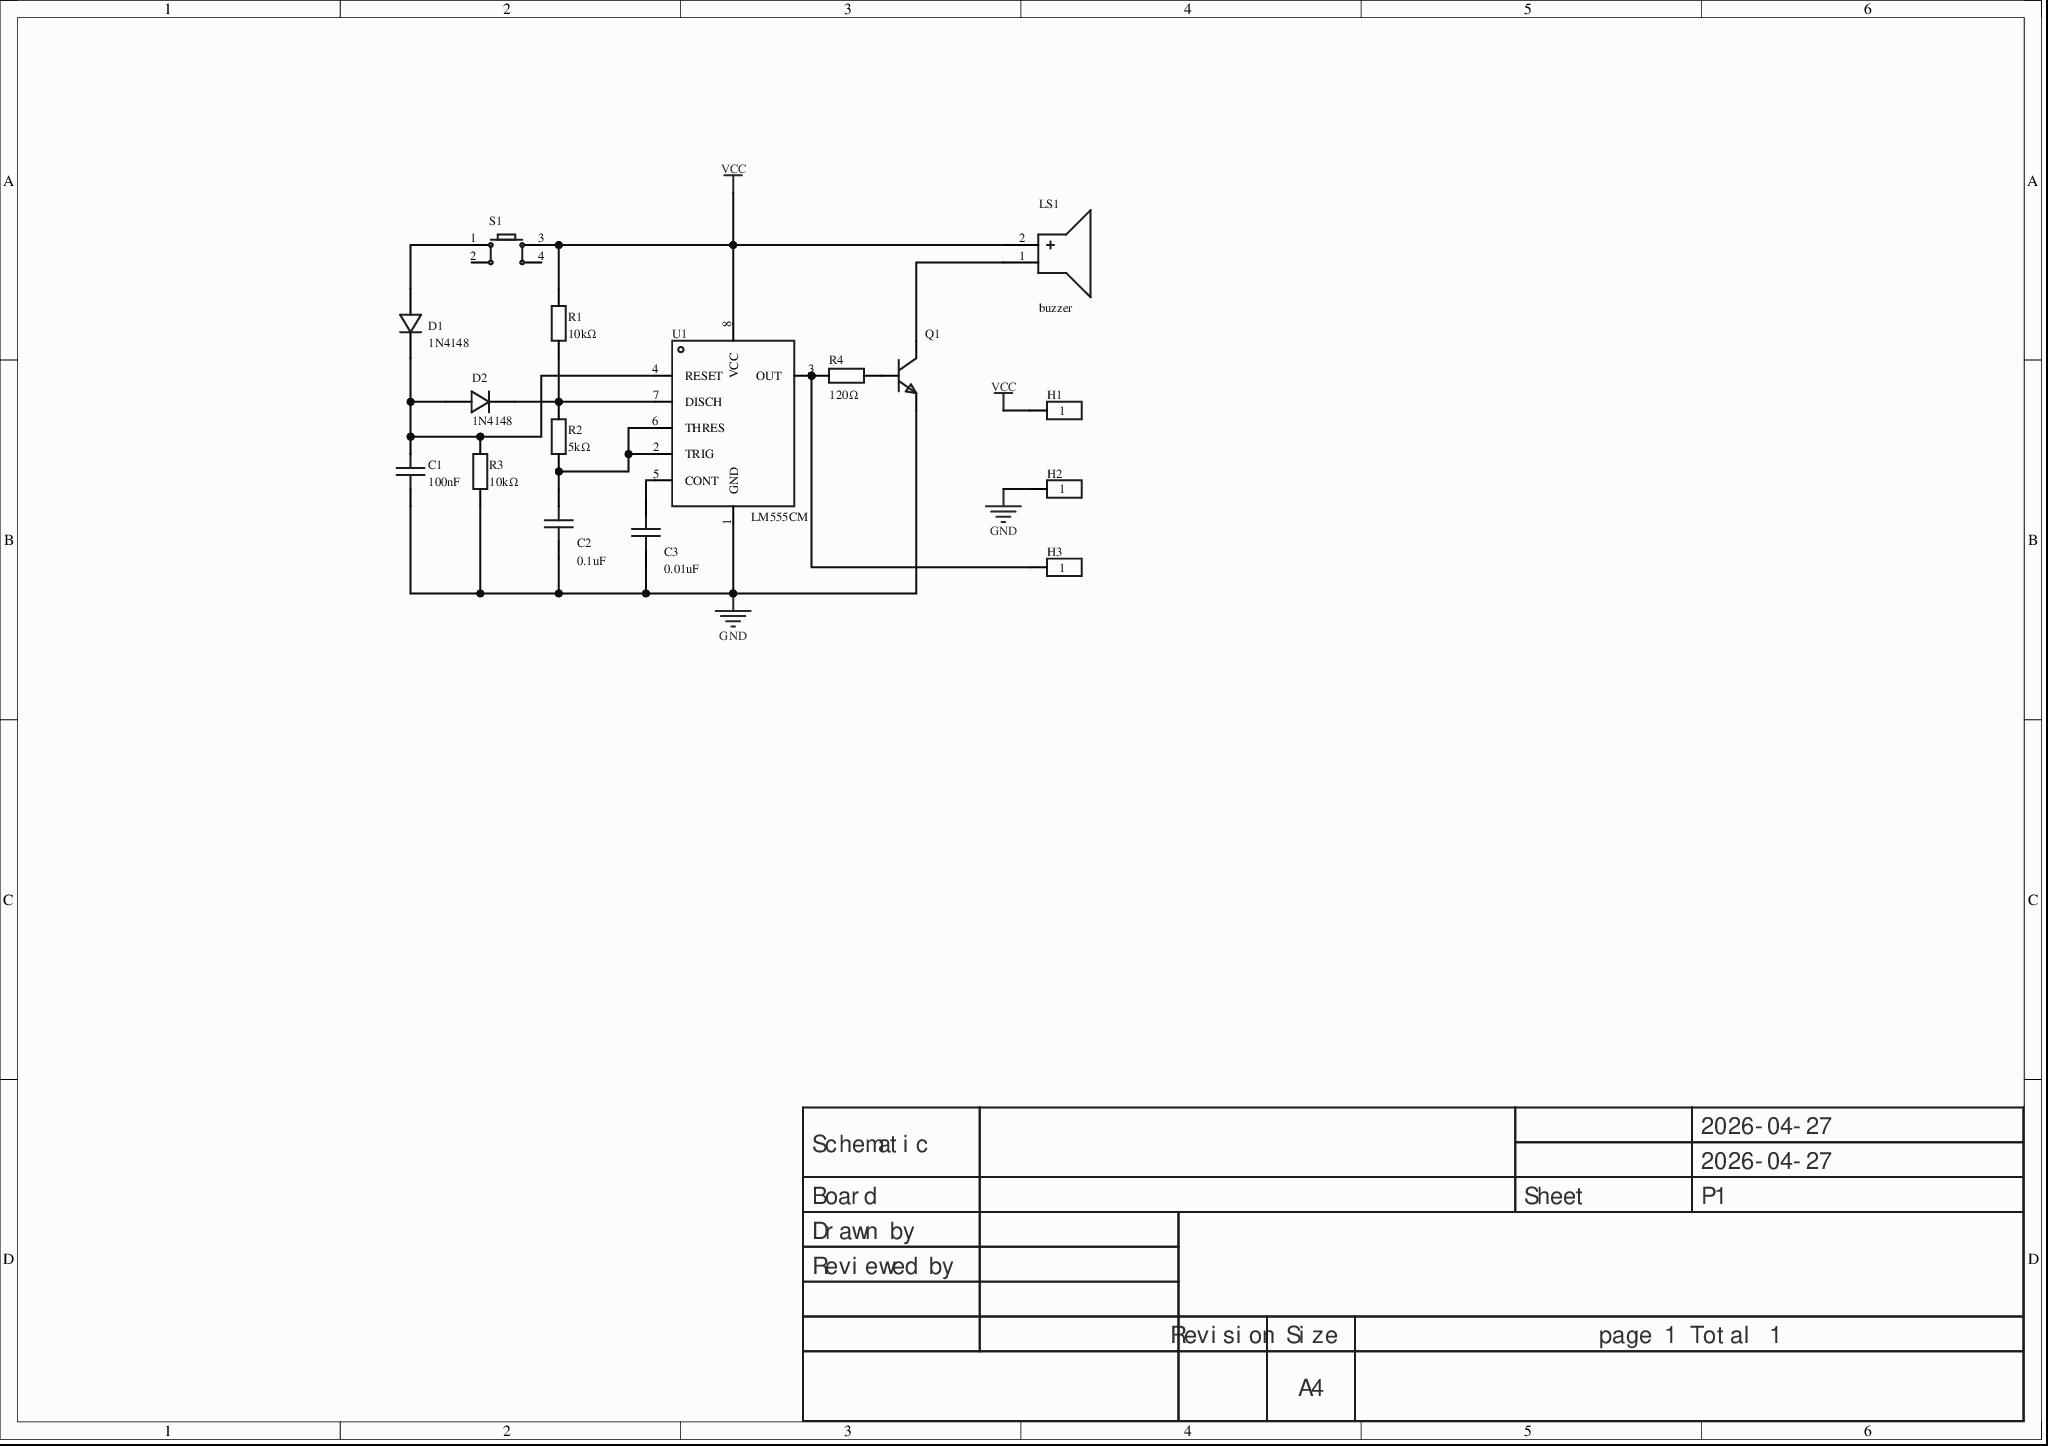
[diagram p0: MISC52004-3.schdoc]
# Altium project MISC52004-2.PrjPcb
1 sheet, 16 parts. Net scope: global (net labels, ports and power ports of the same name join across sheets).
Board file: MISC52004.pcbdoc

## Sheet MISC52004-3.schdoc
size 297 x 209 mm; Version: V1.0; @Project Name: MISC52004; @Update Date: 2026-04-27; @Create Date: 2026-04-27; @Board Name: MISC52004; @Create Time: 22:00:04; @Page Count: 1; @Page No: 1; @Schematic Name: MISC52004; @Update Time: 22:00:04; Size: A4

### Parts
C1  100nF  [CAP-TH_L5.0-W2.5-P5.00-D1.0]
C2  0.1uF  [CAP-TH_L5.0-W2.5-P5.00-D1.0]
C3  0.01uF  [CAP-TH_L5.0-W2.5-P5.00-D1.0]
D1  1N4148  [DO-35_BD2.2-L4.0-D0.50_1N4148]
D2  1N4148  [DO-35_BD2.2-L4.0-D0.50_1N4148]
H1  (no value)  [HDR-TH_1P-V-M_XKB_X4611WV-01I-C28D40]
H2  (no value)  [HDR-TH_1P-V-M_XKB_X4611WV-01I-C28D40]
H3  (no value)  [HDR-TH_1P-V-M_XKB_X4611WV-01I-C28D40]
LS1  buzzer  [BUZ-TH_BD12.0-P6.00-D0.9-RD]
Q1  (no value)  [S8050_TO_92]
R1  10kΩ  [Res_1/8W]
R2  5kΩ  [Res_1/8W]
R3  10kΩ  [Res_1/8W]
R4  120Ω  [Res_1/8W]
S1  (no value)  [SW-TH_4P-L6.0-W6.0-P4.50-LS6.5]
U1  LM555CM  [PDIP-8_L9.6-W6.4-P2.54-LS7.9-BL-1]

### Nets
GND: C1.2 C2.2 C3.2 H2.1 Q1.1(E) R3.1 U1.1(GND)
VCC: H1.1 LS1.2(+) R1.2 S1.3 U1.8(VCC)
NetC1_1: C1.1 D1.2(C) D2.1(A) R3.2 U1.4(RESET)
NetC2_1: C2.1 R2.1 U1.2(TRIG) U1.6(THRES)
NetC3_1: C3.1 U1.5(CONT)
NetD1_1: D1.1(A) S1.1
NetD2_2: D2.2(C) R1.1 R2.2 U1.7(DISCH)
NetH3_1: H3.1 R4.1 U1.3(OUT)
NetLS1_1: LS1.1(-) Q1.3(C)
NetQ1_2: Q1.2(B) R4.2

Not connected (* = marked no-connect by the designer): S1 2 4

### Notes on the sheet
- 2026-04-27
- Schematic
- Board
- Sheet
- P1
- Drawn by
- Reviewed by
- Revision
- Size
- A4
- page 1 Total 1

### Library data of the parts
C1-C3 = 100nF: Symbol: 100NF_C9900015256; AddInBom: yes; ModelId: 08e3d7481fc7486bb1b263873f51e1e10819f05c4eef4c71ace90d822a990e87; ModelName: CAP-TH_BD5.0-W2.5-P5.08; ModelTransform: 224.652,98.425,0,0,0,0,-0.005,0,-137.795; Device: 100nF; LCSC Part Name: 100nF; SupplierPart: C9900015256; Supplier Footprint: CAP-TH_L5.0-W2.5-P5.00-D1.0; JLCPCB Part Class: Extended Part; Supplier: LCSC; ConvertToPcb: yes; FootprintName: CAP-TH_L5.0-W2.5-P5.00-D1.0
  C1: ManufacturerPart: 100nF
  C2: Manufacturer Part: 0.1uF
  C3: Manufacturer Part: 0.01uF
D1 D2 = 1N4148_C9900036548: AddInBom: yes; ModelId: b29439ed7b924f62acded4384188502f0819f05c4eef4c71ace90d822a990e87; ModelTransform: 334.645,87.008,0,0,0,0,0,0,-196.85; Symbol: 1N4148_C9900036548; Device: 1N4148_C9900036548; LCSC Part Name: 1N4148; SupplierPart: C9900036548; ManufacturerPart: 1N4148; Supplier Footprint: LL34; JLCPCB Part Class: Extended Part; Supplier: LCSC; ConvertToPcb: yes; FootprintName: DO-35_BD2.2-L4.0-D0.50_1N4148; ModelName: DO-35_BD2.2-L4.0-D0.50_1N4148
H1-H3 = HDR-M_2.54_1x1P: Symbol: HDR_1x1; ConvertToPcb: yes; ModelId: 95857080d3cc4057a19a22ccce05e1710819f05c4eef4c71ace90d822a990e87; ModelTransform: 78.74,79.1337,0,0,0,0,0,0,-110.236; Device: HDR-M_2.54_1x1P; AddInBom: yes; SupplierPart: C81276; Supplier Footprint: 插件; FootprintName: HDR-TH_1P-V-M_XKB_X4611WV-01I-C28D40; JLCPCB Part Class: Extended Part; ModelName: HDR-TH_1P-V-M_XKB_X4611WV-01I-C28D40
LS1 = buzzer: AddInBom: yes; ModelId: af17e4151ed84fc2a628230bf23763630819f05c4eef4c71ace90d822a990e87; ModelTransform: 472.44,472.176,0,270,0,0,0,0,-196.85; Symbol: BUZZER; Device: buzzer; LCSC Part Name: buzzer; SupplierPart: C9900014030; ManufacturerPart: buzzer; Supplier Footprint: buzzer; JLCPCB Part Class: Extended Part; Supplier: LCSC; ConvertToPcb: yes; FootprintName: BUZ-TH_BD12.0-P6.00-D0.9-RD; ModelName: BUZ-TH_BD12.0-P6.00-D0.9-RD
Q1 = S8050_TO_NPN: ConvertToPcb: yes; ModelId: aafe8e06f2154e7c93506efd0d6632dd0819f05c4eef4c71ace90d822a990e87; ModelName: TO-92-3_L4.9-W3.7-P1.27-L; ModelTransform: 180.78,141.44,417.3,0,0,0,0,0,-200; Symbol: S8050_TO_NPN; Device: S8050_TO_NPN; AddInBom: yes; Supplier Footprint: TO-92; FootprintName: S8050_TO_92
R1-R4 = Res_AXIAL-1/8W: Symbol: Resistor; ConvertToPcb: yes; ModelId: b2b5ae7ae4c642178fe0039925c86a3f0819f05c4eef4c71ace90d822a990e87; ModelName: RES-TH_BD1.8-L3.2-P7.20-D0.4; ModelTransform: 282.86,66.88,253.09,0,0,0,0,0,-191; Device: Res_AXIAL-1/8W; AddInBom: yes; Supplier Footprint: 轴向引线; FootprintName: Res_1/8W
  R1 R3: Value: 10kΩ
  R2: Value: 5kΩ
  R4: Value: 120Ω
S1 = Key_TH_6x6x6: Contact current:50mA;Rated voltage(DC):12V;Insulation resistance:100MΩ;Circuit structure:SPST;Mounting:Through-hole;Button shape:Round button;Button/cap colour:Black;Actuation force:260gf@±30gf;Operating temperature:-25℃~+70℃;Pin style:PC pin;Switch length:6mm;Switch width:6mm;Switch height:6mm;Has bracket:No;; Symbol: Tact switch; AddInBom: yes; ModelId: 20eee248bc684ccd8cbdbb1d0d91ec6f0819f05c4eef4c71ace90d822a990e87; ModelName: SW-TH_4P-L6.0-W6.0-H5.0-LS6.5-P4.50; ModelTransform: 236.22,323.03,0,90,0,0,0,0,-137.795; Device: Key_TH_6x6x6; ConvertToPcb: yes; FootprintName: SW-TH_4P-L6.0-W6.0-P4.50-LS6.5; Supplier Footprint: 插件
U1 = NE555PE4: NE555 single-precision timer; Manufacturer: TI(德州仪器); AddInBom: yes; ModelId: 1b8eaf096e7944deafe216467068c10e0819f05c4eef4c71ace90d822a990e87; ModelTransform: 377.952,318.897,0,0,0,0,0,0,-118.11; Symbol: NE555PE4; Device: NE555PE4; Manufacturer Part: LM555CM; LCSC Part Name: NE555PE4; SupplierPart: C2859604; Supplier Footprint: PDIP-8; JLCPCB Part Class: Extended Part; Supplier: LCSC; ConvertToPcb: yes; FootprintName: PDIP-8_L9.6-W6.4-P2.54-LS7.9-BL-1; ModelName: PDIP-8_L9.6-W6.4-P2.54-LS7.9-BL-1